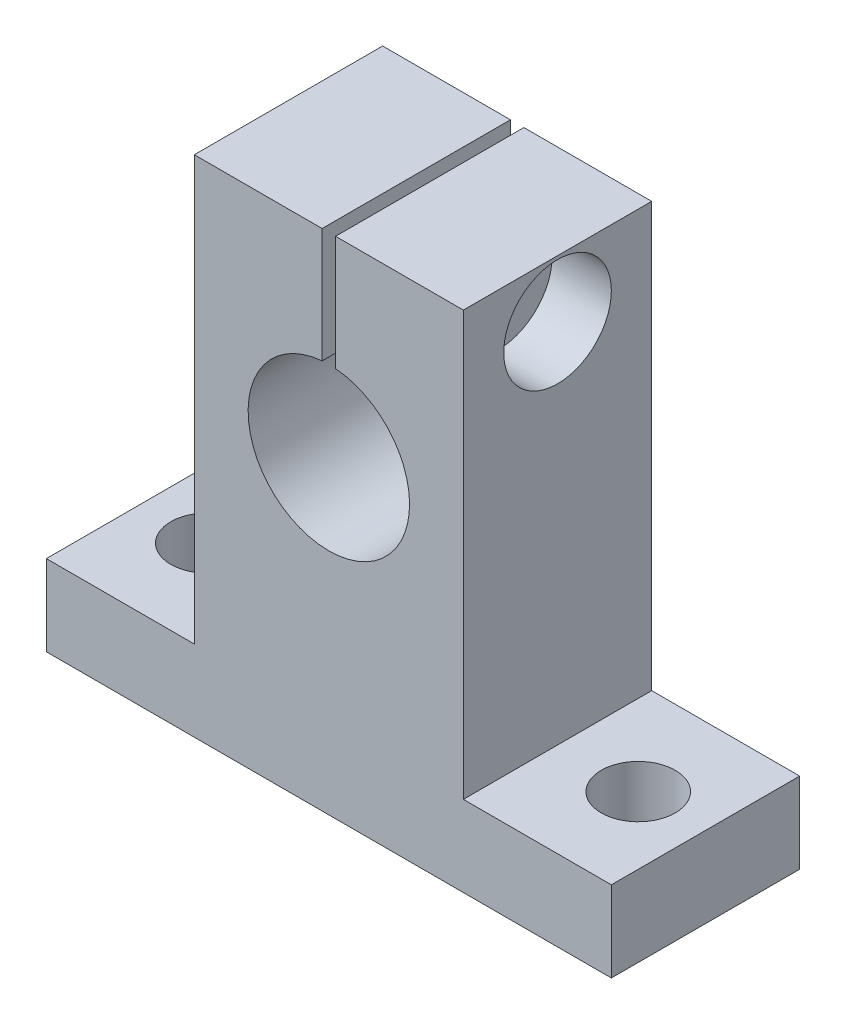
from build123d import *

# Parameters (mm, degrees)
EXTRUDE_1_DEPTH           = 7
HOLE_WIZARD_1_D           = 4.4
HOLE_WIZARD_1_DEPTH       = 9.5
HOLE_WIZARD_1_CBORE_D     = 8
HOLE_WIZARD_1_CBORE_DEPTH = 4.4
HOLE_WIZARD_1_2_D         = 5.5
HOLE_WIZARD_1_3_D         = 3.2


with BuildPart() as part:
    # 草图1 → 凸台-拉伸1 (new, symmetric)
    with BuildSketch(Plane.XY):
        with BuildLine():
            Line((21, 0), (-21, 0))
            Line((-21, 0), (-21, 6))
            Line((-21, 6), (-10, 6))
            Line((-10, 6), (-10, 37.5))
            Line((-10, 37.5), (-0.5, 37.5))
            Line((-0.5, 37.5), (-0.5, 28.979130372))
            ThreePointArc((-0.5, 28.979130372), (0, 17), (0.5, 28.979130372))
            Line((0.5, 28.979130372), (0.5, 37.5))
            Line((0.5, 37.5), (10, 37.5))
            Line((10, 37.5), (10, 6))
            Line((10, 6), (21, 6))
            Line((21, 6), (21, 0))
        make_face()
    extrude(amount=EXTRUDE_1_DEPTH, both=True)

    # Hole Wizard 1
    with Locations(Plane(origin=(10, 0, 0), x_dir=(0, 0, -1), z_dir=(1, 0, 0))):
        with Locations((0, 33.25)):
            CounterBoreHole(HOLE_WIZARD_1_D / 2, HOLE_WIZARD_1_CBORE_D / 2, HOLE_WIZARD_1_CBORE_DEPTH, depth=HOLE_WIZARD_1_DEPTH)

    # Hole Wizard 1 2 (through all)
    with Locations(Plane(origin=(0, 6, 0), x_dir=(1, 0, 0), z_dir=(0, 1, 0))):
        with Locations((-16, 0), (16, 0)):
            Hole(HOLE_WIZARD_1_2_D / 2)

    # Hole Wizard 1 3 (through all)
    with Locations(Plane(origin=(-0.5, 0, 0), x_dir=(0, 0, -1), z_dir=(1, 0, 0))):
        with Locations((0, 33.25)):
            Hole(HOLE_WIZARD_1_3_D / 2)


solid = part.part
